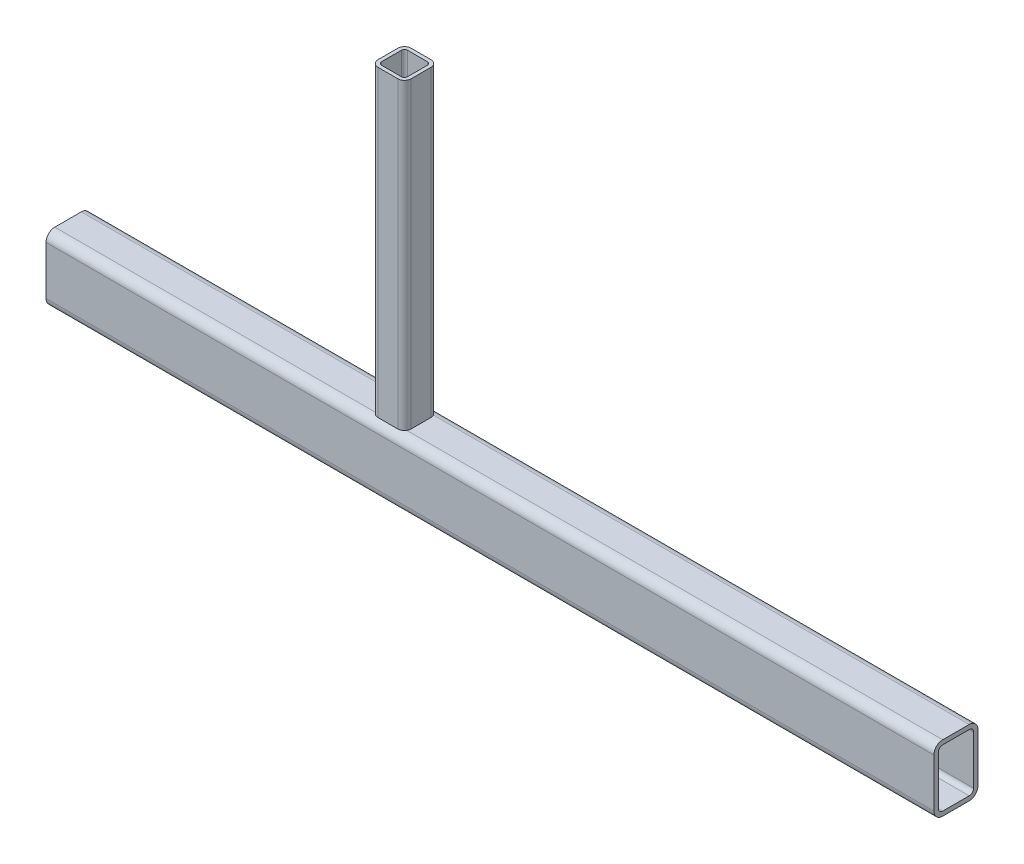
from build123d import *

# Parameters (mm, degrees)
GB_T_6728_2002_RECTANGULAR_HOLLOW_SECTIO_DEPTH = 805
GB_T_6728_2002_SQUARE_HOLLOW_SECTION_30_DEPTH  = 305


with BuildPart() as part:
    # Sketch12 → GB/T 6728-2002 rectangular hollow section 60X40X4(1) (new body)
    with BuildSketch(Plane(origin=(0, 0, 0), x_dir=(0, 0, 1), z_dir=(1, 0, 0))):
        with BuildLine():
            Line((-12, -30), (12, -30))
            ThreePointArc((12, -30), (17.656854249, -27.656854249), (20, -22))
            Line((20, -22), (20, 22))
            ThreePointArc((20, 22), (17.656854249, 27.656854249), (12, 30))
            Line((12, 30), (-12, 30))
            ThreePointArc((-12, 30), (-17.656854249, 27.656854249), (-20, 22))
            Line((-20, 22), (-20, -22))
            ThreePointArc((-20, -22), (-17.656854249, -27.656854249), (-12, -30))
        make_face()
        with BuildLine():
            Line((-12, -26), (12, -26))
            ThreePointArc((12, -26), (14.828427125, -24.828427125), (16, -22))
            Line((16, -22), (16, 22))
            ThreePointArc((16, 22), (14.828427125, 24.828427125), (12, 26))
            Line((12, 26), (-12, 26))
            ThreePointArc((-12, 26), (-14.828427125, 24.828427125), (-16, 22))
            Line((-16, 22), (-16, -22))
            ThreePointArc((-16, -22), (-14.828427125, -24.828427125), (-12, -26))
        make_face(mode=Mode.SUBTRACT)
    extrude(amount=GB_T_6728_2002_RECTANGULAR_HOLLOW_SECTIO_DEPTH)


with BuildPart() as body_2:
    # Sketch16 → GB/T 6728-2002 square hollow section 30×3.2(1) (new body)
    with BuildSketch(Plane(origin=(305, 0, 0), x_dir=(-1, 0, 0), z_dir=(0, 1, 0))):
        with BuildLine():
            Line((-9, -15), (9, -15))
            ThreePointArc((9, -15), (13.242640687, -13.242640687), (15, -9))
            Line((15, -9), (15, 9))
            ThreePointArc((15, 9), (13.242640687, 13.242640687), (9, 15))
            Line((9, 15), (-9, 15))
            ThreePointArc((-9, 15), (-13.242640687, 13.242640687), (-15, 9))
            Line((-15, 9), (-15, -9))
            ThreePointArc((-15, -9), (-13.242640687, -13.242640687), (-9, -15))
        make_face()
        with BuildLine():
            Line((-9, -11.8), (9, -11.8))
            ThreePointArc((9, -11.8), (10.979898987, -10.979898987), (11.8, -9))
            Line((11.8, -9), (11.8, 9))
            ThreePointArc((11.8, 9), (10.979898987, 10.979898987), (9, 11.8))
            Line((9, 11.8), (-9, 11.8))
            ThreePointArc((-9, 11.8), (-10.979898987, 10.979898987), (-11.8, 9))
            Line((-11.8, 9), (-11.8, -9))
            ThreePointArc((-11.8, -9), (-10.979898987, -10.979898987), (-9, -11.8))
        make_face(mode=Mode.SUBTRACT)
    extrude(amount=GB_T_6728_2002_SQUARE_HOLLOW_SECTION_30_DEPTH)

    # Trim_Extend1 9
    split(bisect_by=Plane(origin=(402.5, 30, 0), x_dir=(-1, 0, 0), z_dir=(0, 1, 0)), keep=Keep.TOP)


solid = Compound([part.part, body_2.part])
